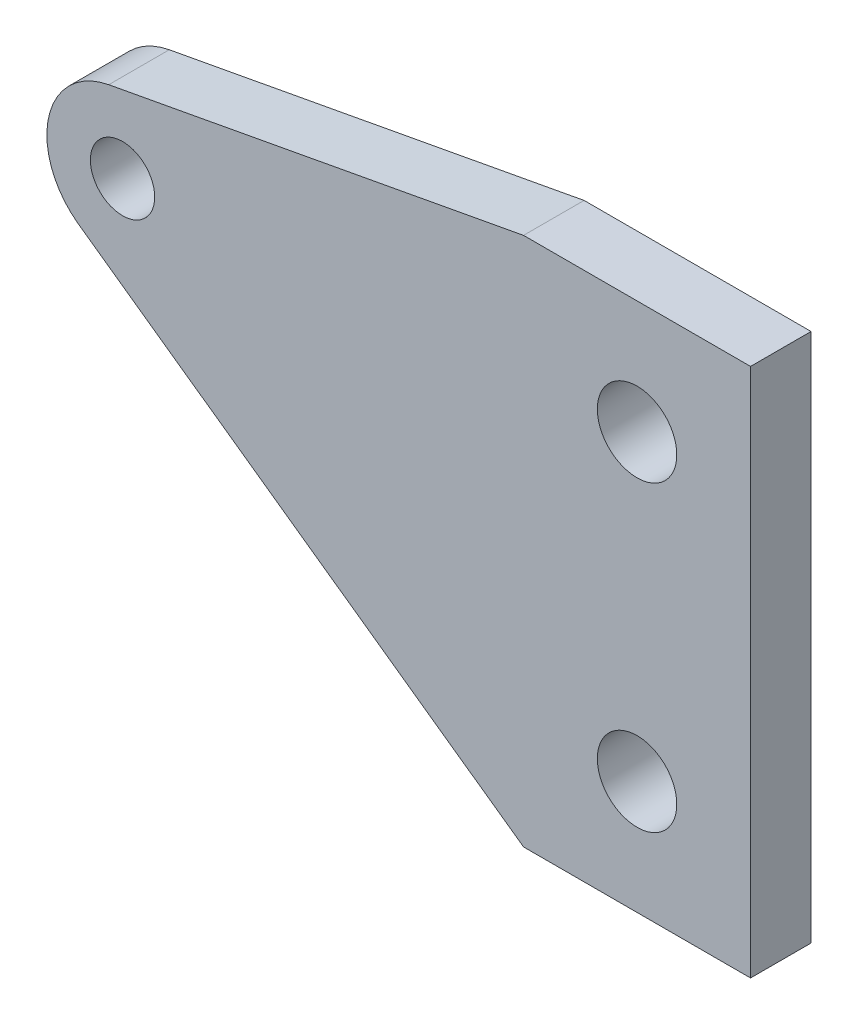
from build123d import *

# Parameters (mm, degrees)
SKETCH1_W              = 100
SKETCH1_H              = 70
SKETCH1_R              = 5.25
BOSS_EXTRUDE1_DEPTH    = 8
SKETCH2_OUTSIDE_W      = 126.466
SKETCH2_OUTSIDE_H      = 96.466
CUT_EXTRUDE1_DEPTH     = 10
M10_TAPPED_HOLE1_D     = 8.5
M10_TAPPED_HOLE1_DEPTH = 24.5
M10_TAPPED_HOLE1_TIP   = 2.553657631


with BuildPart() as part:
    # Sketch1 → Boss-Extrude1 (new body)
    with BuildSketch(Plane.XY.offset(4)):
        with Locations((5.613636364, -1.590909091)):
            Rectangle(SKETCH1_W, SKETCH1_H)
        with Locations(Location((40.613636364, -21.590909091, 0), (0, 0, 180))):
            Circle(SKETCH1_R, mode=Mode.SUBTRACT)
        with Locations(Location((40.613636364, 18.409090909, 0), (0, 0, 180))):
            Circle(SKETCH1_R, mode=Mode.SUBTRACT)
    extrude(amount=-BOSS_EXTRUDE1_DEPTH)

    # Sketch2 outside → Cut-Extrude1 (cut)
    with BuildSketch(Plane.XY.offset(4)):
        with Locations((5.614, -1.591)):
            Rectangle(SKETCH2_OUTSIDE_W, SKETCH2_OUTSIDE_H)
        with BuildLine():
            Line((25.613636364, 33.409090909), (-29.209885446, 23.241423705))
            ThreePointArc((-29.209885446, 23.241423705), (-37.150522341, 15.56807326), (-33.185327877, 5.262188814))
            Line((-33.185327877, 5.262188814), (25.613636364, -36.590909091))
            Line((25.613636364, -36.590909091), (55.613636364, -36.590909091))
            Line((55.613636364, -36.590909091), (55.613636364, 33.409090909))
            Line((55.613636364, 33.409090909), (25.613636364, 33.409090909))
        make_face(mode=Mode.SUBTRACT)
    extrude(amount=-CUT_EXTRUDE1_DEPTH, mode=Mode.SUBTRACT)

    # M10 Tapped Hole1
    with Locations(Plane.XY.offset(4)):
        with Locations((-27.386363636, 13.409090909)):
            Hole(M10_TAPPED_HOLE1_D / 2, depth=M10_TAPPED_HOLE1_DEPTH)
            with Locations((0, 0, -(M10_TAPPED_HOLE1_DEPTH + M10_TAPPED_HOLE1_TIP / 2))):  # 118° drill point
                Cone(0, M10_TAPPED_HOLE1_D / 2, M10_TAPPED_HOLE1_TIP, mode=Mode.SUBTRACT)


solid = part.part
